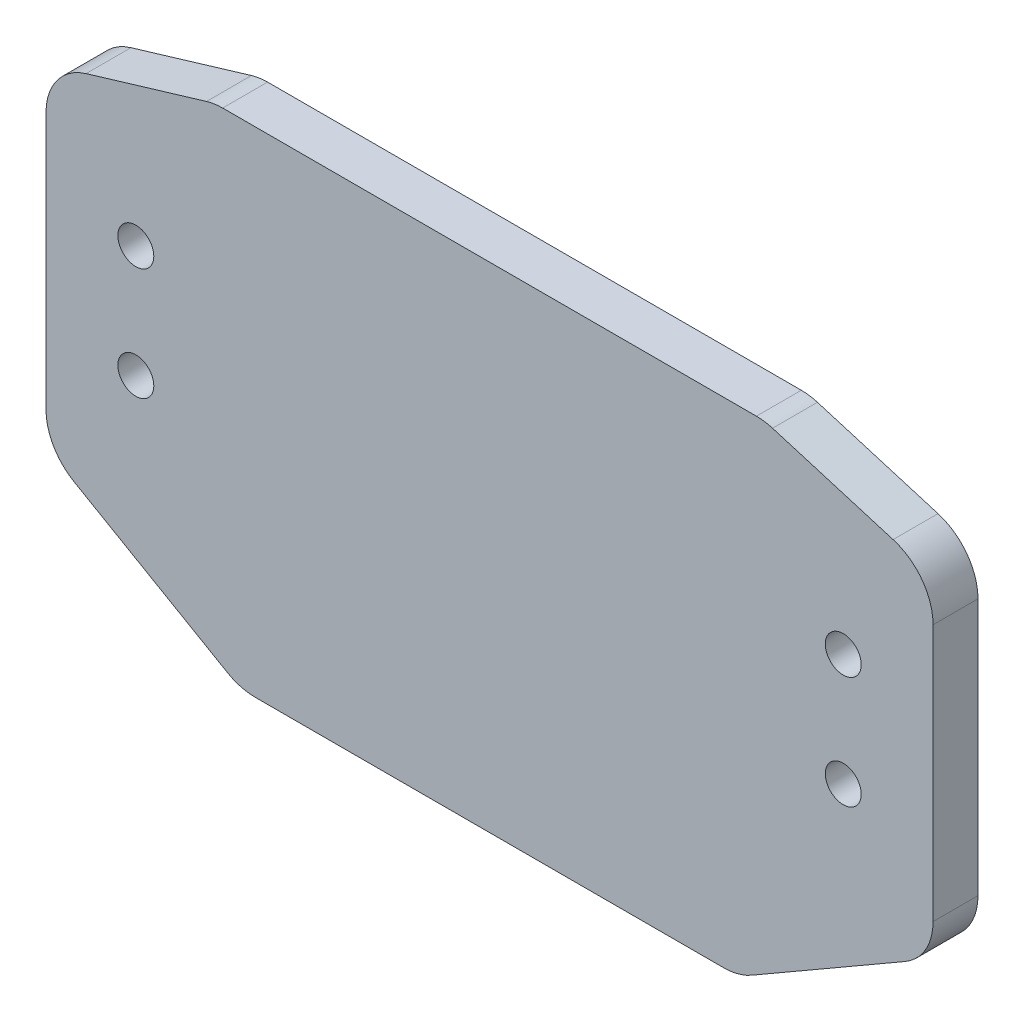
from build123d import *

# Parameters (mm, degrees)
SKETCH_1_R      = 1.6
EXTRUDE_1_DEPTH = 4
FILLET_R5_1_R   = 5


with BuildPart() as part:
    # 草图1 → 凸台-拉伸1 (new body)
    with BuildSketch(Plane.XY):
        Polygon((-24.5, 23.5), (24.5, 23.5), (39.5, 19), (39.5, -10.5), (22.179491924, -20.5), (-22.179491924, -20.5), (-39.5, -10.5), (-39.5, 19), align=None)
        with Locations((-31.5, 9)):
            Circle(SKETCH_1_R, mode=Mode.SUBTRACT)
        with Locations((-31.5, -1)):
            Circle(SKETCH_1_R, mode=Mode.SUBTRACT)
        with Locations(Location((31.5, -1, 0), (0, 0, 180))):
            Circle(SKETCH_1_R, mode=Mode.SUBTRACT)
        with Locations(Location((31.5, 9, 0), (0, 0, 180))):
            Circle(SKETCH_1_R, mode=Mode.SUBTRACT)
    extrude(amount=EXTRUDE_1_DEPTH)

    # R5 圆角1
    fillet_r5_1_edges = [part.edges().sort_by_distance(p)[0] for p in [
        (-24.5, 23.5, 2),
        (24.5, 23.5, 2),
        (39.5, 19, 2),
        (39.5, -10.5, 2),
        (22.179491924, -20.5, 2),
        (-22.179491924, -20.5, 2),
        (-39.5, -10.5, 2),
        (-39.5, 19, 2),
    ]]
    fillet(fillet_r5_1_edges, radius=FILLET_R5_1_R)


solid = part.part
